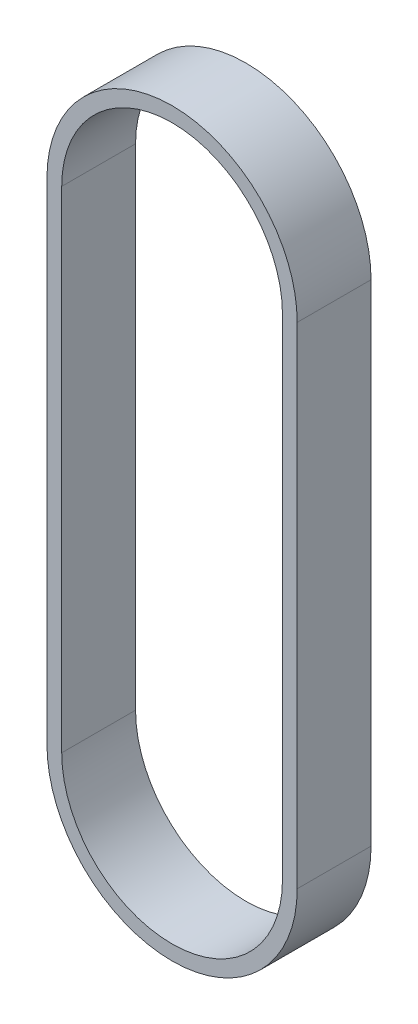
SolidWorks part; units mm, degrees
ref_plane "Front Plane" through (0, 0, 0) normal (0, 0, 1) x (1, 0, 0)
ref_plane "Top Plane" through (0, 0, 0) normal (0, 1, 0) x (1, 0, 0)
ref_plane "Right Plane" through (0, 0, 0) normal (1, 0, 0) x (0, 0, -1)
sketch "Sketch2" plane through (0, 0, 0) normal (0, 0, 1) x (1, 0, 0)
  line L0 (0, 0) -> (1, 0) construction
  line L1 (0, 0) -> (0, 1) construction
  line L2 (3.5482, -3.0006) -> (3.5482, -69.4256)
  line L3 (-30.3418, -69.4256) -> (-30.3418, -3.0006)
  arc A0 (-30.3418, -3.0006) -> (3.5482, -3.0006) centre (-13.3968, -3.0006) cw
  arc A1 (3.5482, -69.4256) -> (-30.3418, -69.4256) centre (-13.3968, -69.4256) cw
extrude "Extrude-Thin1" add sketch "Sketch2" along normal blind 10 thin
